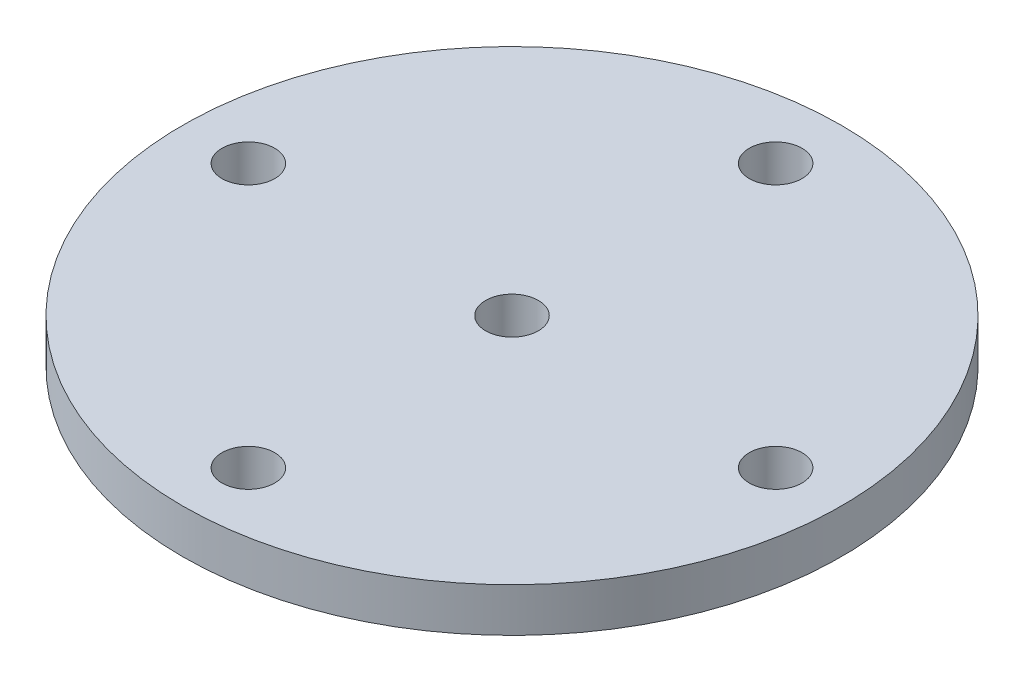
from build123d import *

# Parameters (mm, degrees)
SKETCH1_R           = 75
BOSS_EXTRUDE1_DEPTH = 10
SKETCH2_R           = 6
CUT_EXTRUDE1_DEPTH  = 107.536378763


with BuildPart() as part:
    # Sketch1 → Boss-Extrude1 (new body)
    with BuildSketch(Plane(origin=(0, 0, 0), x_dir=(1, 0, 0), z_dir=(0, 1, 0))):
        with Locations(Location((0, 0, 0), (0, 0, 270))):
            Circle(SKETCH1_R)
    extrude(amount=BOSS_EXTRUDE1_DEPTH)

    # Sketch2 → Cut-Extrude1 (cut, through all)
    with BuildSketch(Plane(origin=(0, 10, 0), x_dir=(1, 0, 0), z_dir=(0, 1, 0))):
        with Locations(Location((0, 60, 0), (0, 0, 270))):
            Circle(SKETCH2_R)
        with Locations(Location((0, 0, 0), (0, 0, 270))):
            Circle(SKETCH2_R)
        with Locations(Location((0, -60, 0), (0, 0, 270))):
            Circle(SKETCH2_R)
        with Locations(Location((-60, 0, 0), (0, 0, 270))):
            Circle(SKETCH2_R)
        with Locations(Location((60, 0, 0), (0, 0, 270))):
            Circle(SKETCH2_R)
    extrude(amount=-CUT_EXTRUDE1_DEPTH, mode=Mode.SUBTRACT)


solid = part.part
